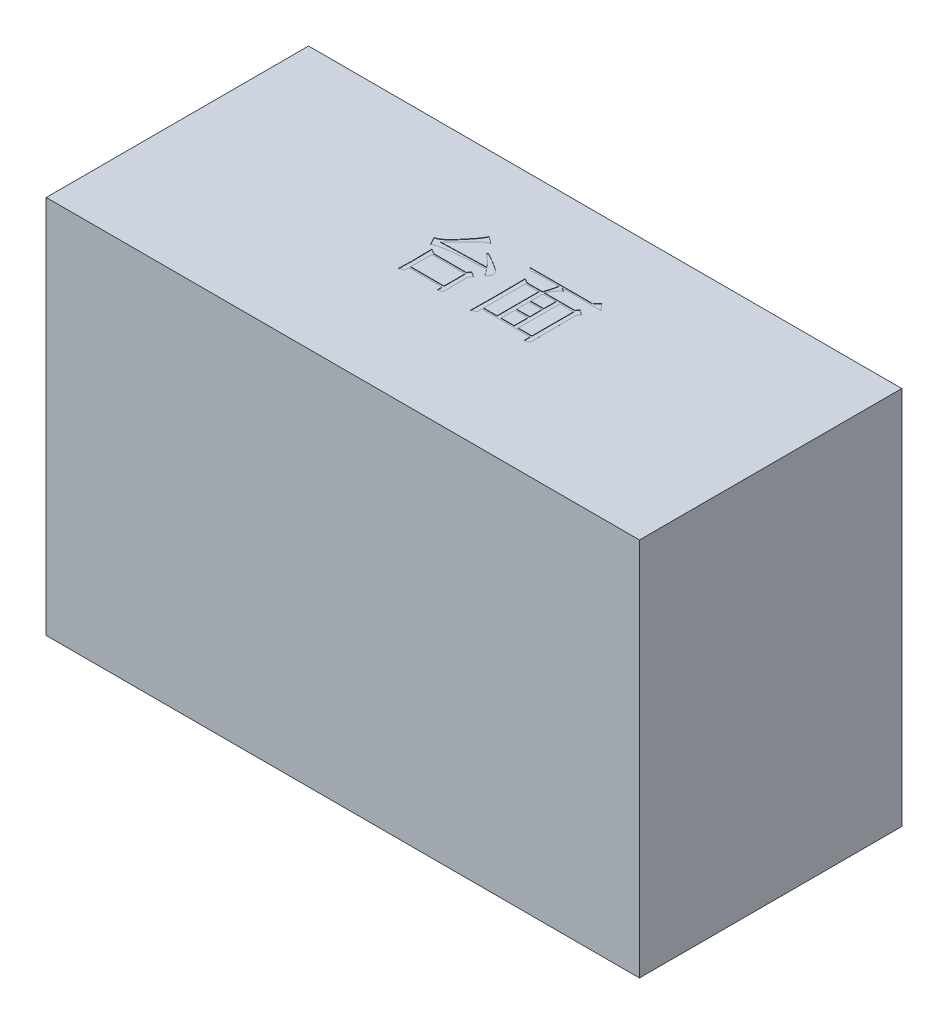
SolidWorks part; units mm, degrees
ref_plane "前视基准面" through (0, 0, 0) normal (0, 0, 1) x (1, 0, 0)
ref_plane "上视基准面" through (0, 0, 0) normal (0, 1, 0) x (1, 0, 0)
ref_plane "右视基准面" through (0, 0, 0) normal (1, 0, 0) x (0, 0, -1)
other "Configuration Table"
sketch "草图1" plane through (0, 0, 0) normal (0, 0, 1) x (1, 0, 0)
  line L1 (-735, 470) -> (735, 470)
  line L2 (-735, 470) -> (-735, -470)
  line L3 (-735, -470) -> (735, -470)
  line L4 (735, 470) -> (735, -470)
  line L5 (-735, 470) -> (735, -470) construction
  line L6 (-735, -470) -> (735, 470) construction
  point P0 (0, 0)
  dimension "D1" = 1470
  dimension "D2" = 940
extrude "凸台-拉伸1" add sketch "草图1" along normal blind 650
sketch "草图2" plane through (0, 470, 0) normal (0, 1, 0) x (1, 0, 0)
  text T0 "台面" font "宋体" height 133.5
extrude "切除-拉伸1" cut sketch "草图2" against normal blind 1
